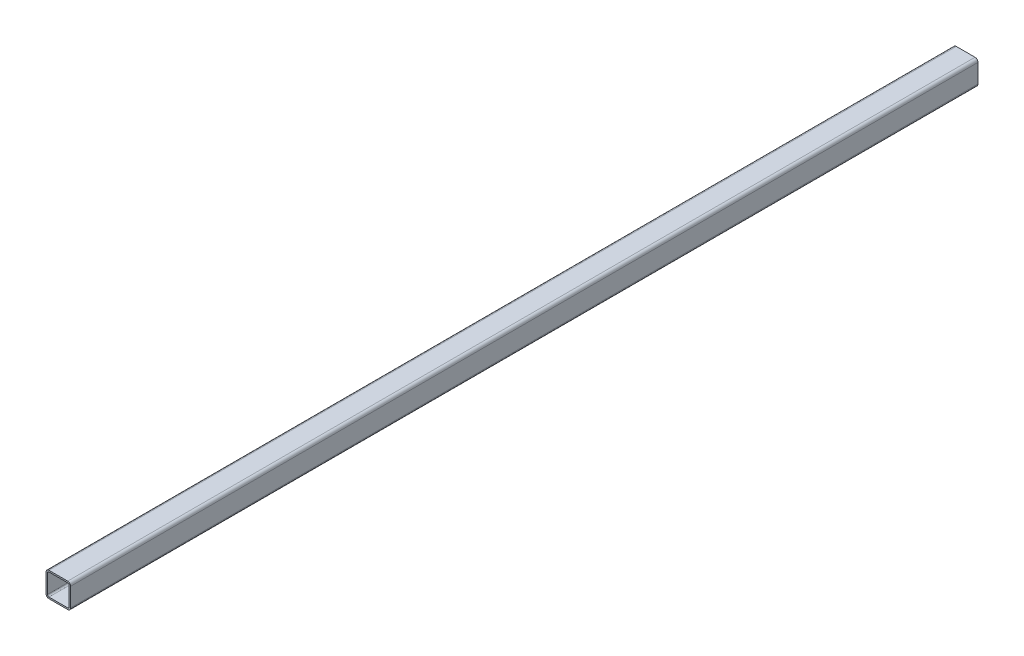
from build123d import *

# Parameters (mm, degrees)
GB_6728_1986_050_X_50_X_3_1_DEPTH = 1840


with BuildPart() as part:
    # Sketch1 → Gb／6728-1986方形空心型钢 050 X 50 X 3(1) (new body)
    with BuildSketch(Plane.YX.offset(-920)):
        with BuildLine():
            Line((-19, -25), (19, -25))
            ThreePointArc((19, -25), (23.242640687, -23.242640687), (25, -19))
            Line((25, -19), (25, 19))
            ThreePointArc((25, 19), (23.242640687, 23.242640687), (19, 25))
            Line((19, 25), (-19, 25))
            ThreePointArc((-19, 25), (-23.242640687, 23.242640687), (-25, 19))
            Line((-25, 19), (-25, -19))
            ThreePointArc((-25, -19), (-23.242640687, -23.242640687), (-19, -25))
        make_face()
        with BuildLine():
            Line((-19, -22), (19, -22))
            ThreePointArc((19, -22), (21.121320344, -21.121320344), (22, -19))
            Line((22, -19), (22, 19))
            ThreePointArc((22, 19), (21.121320344, 21.121320344), (19, 22))
            Line((19, 22), (-19, 22))
            ThreePointArc((-19, 22), (-21.121320344, 21.121320344), (-22, 19))
            Line((-22, 19), (-22, -19))
            ThreePointArc((-22, -19), (-21.121320344, -21.121320344), (-19, -22))
        make_face(mode=Mode.SUBTRACT)
    extrude(amount=GB_6728_1986_050_X_50_X_3_1_DEPTH)


solid = part.part
